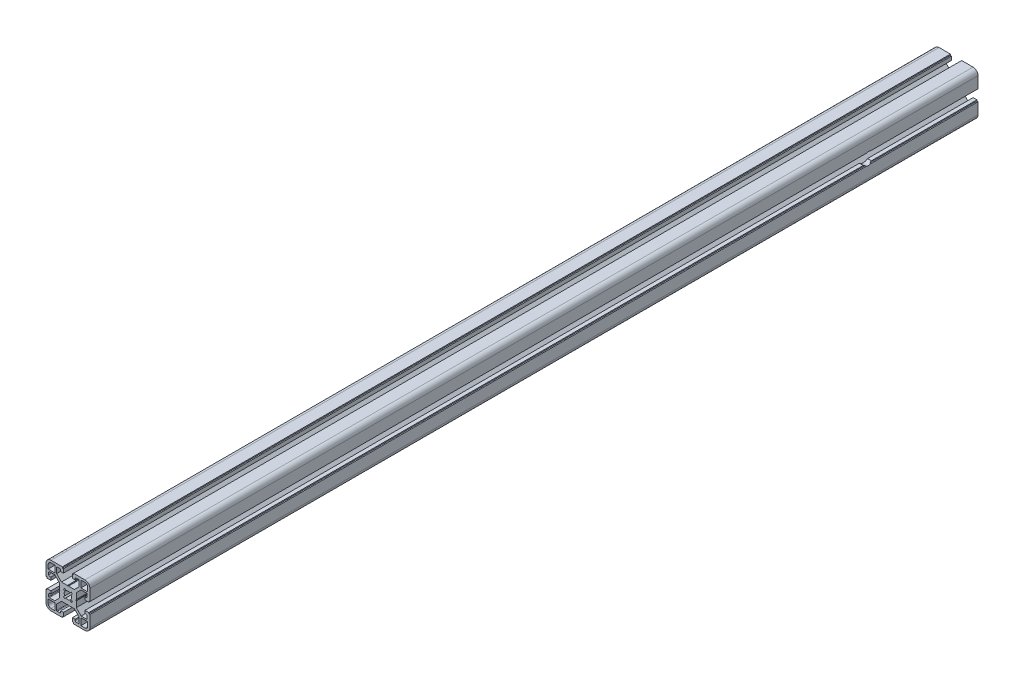
SolidWorks part; units mm, degrees
material "6061 GB/T6892-2006"
ref_plane "前视" through (0, 0, 0) normal (0, 0, 1) x (1, 0, 0)
ref_plane "上视" through (0, 0, 0) normal (0, 1, 0) x (1, 0, 0)
ref_plane "右视" through (0, 0, 0) normal (1, 0, 0) x (0, 0, -1)
sketch "草图1" plane through (0, 0, 0) normal (0, 0, 1) x (1, 0, 0)
  line L0 (-18.9995, -4.1003) -> (-18.9995, -5.1003)
  line L1 (-18.9995, -5.1003) -> (-19.9995, -5.1003)
  line L2 (-19.9995, -5.1003) -> (-19.9995, -15.5003)
  line L3 (-15.4995, -20.0003) -> (-5.0995, -20.0003)
  line L4 (-5.0995, -20.0003) -> (-5.0995, -19.0003)
  line L5 (-5.0995, -19.0003) -> (-4.0995, -19.0003)
  line L6 (-4.0995, -19.0003) -> (-4.0995, -15.5003)
  line L7 (-4.0995, -15.5003) -> (-6.5995, -15.5003)
  line L8 (-6.5995, -15.5003) -> (-6.5995, -16.5003)
  line L9 (-7.5995, -17.5003) -> (-9.7995, -17.5003)
  line L10 (-10.2995, -17.0003) -> (-10.2995, -11.9973)
  line L11 (-10.2995, -11.9973) -> (-5.9025, -7.6003)
  line L12 (-5.9025, -7.6003) -> (-0.5195, -7.6003)
  line L13 (-0.5195, -7.6003) -> (0.0005, -7.3003)
  line L14 (0.0005, -7.3003) -> (0.5195, -7.6003)
  line L15 (0.5195, -7.6003) -> (5.9035, -7.6003)
  line L16 (5.9035, -7.6003) -> (10.3005, -11.9973)
  line L17 (10.3005, -11.9973) -> (10.3005, -17.0003)
  line L18 (9.8005, -17.5003) -> (7.6005, -17.5003)
  line L19 (6.6005, -16.5003) -> (6.6005, -15.5003)
  line L20 (6.6005, -15.5003) -> (4.1005, -15.5003)
  line L21 (4.1005, -15.5003) -> (4.1005, -19.0003)
  line L22 (4.1005, -19.0003) -> (5.1005, -19.0003)
  line L23 (5.1005, -19.0003) -> (5.1005, -20.0003)
  line L24 (5.1005, -20.0003) -> (15.5005, -20.0003)
  line L25 (20.0005, -15.5003) -> (20.0005, -5.1003)
  line L26 (20.0005, -5.1003) -> (19.0005, -5.1003)
  line L27 (19.0005, -5.1003) -> (19.0005, -4.1003)
  line L28 (19.0005, -4.1003) -> (15.5005, -4.1003)
  line L29 (15.5005, -4.1003) -> (15.5005, -6.6003)
  line L30 (15.5005, -6.6003) -> (16.5005, -6.6003)
  line L31 (17.5005, -7.6003) -> (17.5005, -9.8003)
  line L32 (17.0005, -10.3003) -> (11.9975, -10.3003)
  line L33 (11.9975, -10.3003) -> (7.6005, -5.9033)
  line L34 (7.6005, -5.9033) -> (7.6005, -0.5203)
  line L35 (7.6005, -0.5203) -> (7.3005, -0.0003)
  line L36 (7.3005, -0.0003) -> (7.6005, 0.5197)
  line L37 (7.6005, 0.5197) -> (7.6005, 5.9027)
  line L38 (7.6005, 5.9027) -> (11.9975, 10.2997)
  line L39 (11.9975, 10.2997) -> (17.0005, 10.2997)
  line L40 (17.5005, 9.7997) -> (17.5005, 7.5997)
  line L41 (16.5005, 6.5997) -> (15.5005, 6.5997)
  line L42 (15.5005, 6.5997) -> (15.5005, 4.0997)
  line L43 (15.5005, 4.0997) -> (19.0005, 4.0997)
  line L44 (19.0005, 4.0997) -> (19.0005, 5.0997)
  line L45 (19.0005, 5.0997) -> (20.0005, 5.0997)
  line L46 (20.0005, 5.0997) -> (20.0005, 15.4997)
  line L47 (15.5005, 19.9997) -> (5.1005, 19.9997)
  line L48 (5.1005, 19.9997) -> (5.1005, 18.9997)
  line L49 (5.1005, 18.9997) -> (4.1005, 18.9997)
  line L50 (4.1005, 18.9997) -> (4.1005, 15.4997)
  line L51 (4.1005, 15.4997) -> (6.6005, 15.4997)
  line L52 (7.6005, 17.4997) -> (9.8005, 17.4997)
  line L53 (10.3005, 16.9997) -> (10.3005, 11.9967)
  line L54 (10.3005, 11.9967) -> (5.9035, 7.5997)
  line L55 (5.9035, 7.5997) -> (0.5195, 7.5997)
  line L56 (0.5195, 7.5997) -> (0.0005, 7.2997)
  line L57 (0.0005, 7.2997) -> (-0.5195, 7.5997)
  line L58 (-0.5195, 7.5997) -> (-5.9025, 7.5997)
  line L59 (-5.9025, 7.5997) -> (-10.2995, 11.9967)
  line L60 (-10.2995, 11.9967) -> (-10.2995, 16.9997)
  line L61 (-9.7995, 17.4997) -> (-7.5995, 17.4997)
  line L62 (-6.5995, 16.4997) -> (-6.5995, 15.4997)
  line L63 (-6.5995, 15.4997) -> (-4.0995, 15.4997)
  line L64 (-4.0995, 15.4997) -> (-4.0995, 18.9997)
  line L65 (-4.0995, 18.9997) -> (-5.0995, 18.9997)
  line L66 (-5.0995, 18.9997) -> (-5.0995, 19.9997)
  line L67 (-5.0995, 19.9997) -> (-15.4995, 19.9997)
  line L68 (-19.9995, 15.4997) -> (-19.9995, 5.0997)
  line L69 (-19.9995, 5.0997) -> (-18.9995, 5.0997)
  line L70 (-18.9995, 5.0997) -> (-18.9995, 4.0997)
  line L71 (-18.9995, 4.0997) -> (-15.4995, 4.0997)
  line L72 (-15.4995, 4.0997) -> (-15.4995, 6.5997)
  line L73 (-15.4995, 6.5997) -> (-16.4995, 6.5997)
  line L74 (-17.4995, 7.5997) -> (-17.4995, 9.7997)
  line L75 (-16.9995, 10.2997) -> (-11.9965, 10.2997)
  line L76 (-11.9965, 10.2997) -> (-7.5995, 5.9027)
  line L77 (-7.5995, 5.9027) -> (-7.5995, 0.5197)
  line L78 (-7.5995, 0.5197) -> (-7.2995, -0.0003)
  line L79 (-7.2995, -0.0003) -> (-7.5995, -0.5203)
  line L80 (-7.5995, -0.5203) -> (-7.5995, -5.9033)
  line L81 (-7.5995, -5.9033) -> (-11.9965, -10.3003)
  line L82 (-11.9965, -10.3003) -> (-16.9995, -10.3003)
  line L83 (-17.4995, -9.8003) -> (-17.4995, -7.6003)
  line L84 (-16.4995, -6.6003) -> (-15.4995, -6.6003)
  line L85 (-15.4995, -6.6003) -> (-15.4995, -4.1003)
  line L86 (-15.4995, -4.1003) -> (-18.9995, -4.1003)
  line L87 (15.5005, -18.0003) -> (11.8005, -18.0003)
  line L88 (11.8005, -18.0003) -> (11.8005, -11.8003)
  line L89 (11.8005, -11.8003) -> (18.0005, -11.8003)
  line L90 (18.0005, -11.8003) -> (18.0005, -15.5003)
  line L91 (18.0005, 11.7997) -> (11.8005, 11.7997)
  line L92 (11.8005, 11.7997) -> (11.8005, 17.9997)
  line L93 (11.8005, 17.9997) -> (15.5005, 17.9997)
  line L94 (18.0005, 15.4997) -> (18.0005, 11.7997)
  line L95 (-1.8145, -2.8753) -> (-3.0044, -4.0665)
  line L96 (-3.0044, -4.0665) -> (-4.0656, -3.0052)
  line L97 (-4.0656, -3.0052) -> (-2.8745, -1.8153)
  line L98 (-2.8745, 1.8147) -> (-4.0644, 3.0058)
  line L99 (-4.0644, 3.0058) -> (-3.0044, 4.0658)
  line L100 (-3.0044, 4.0658) -> (-1.8145, 2.8747)
  line L101 (1.8145, 2.8747) -> (3.0055, 4.0657)
  line L102 (3.0055, 4.0657) -> (4.0666, 3.0045)
  line L103 (4.0666, 3.0045) -> (2.8755, 1.8147)
  line L104 (2.8755, -1.8153) -> (4.0666, -3.0052)
  line L105 (4.0666, -3.0052) -> (3.0055, -4.0663)
  line L106 (3.0055, -4.0663) -> (1.8145, -2.8753)
  line L107 (-17.9995, -15.5003) -> (-17.9995, -11.8003)
  line L108 (-17.9995, -11.8003) -> (-11.7995, -11.8003)
  line L109 (-11.7995, -11.8003) -> (-11.7995, -18.0003)
  line L110 (-11.7995, -18.0003) -> (-15.4995, -18.0003)
  line L111 (-11.7995, 17.9997) -> (-11.7995, 11.7997)
  line L112 (-11.7995, 11.7997) -> (-17.9995, 11.7997)
  line L113 (-17.9995, 11.7997) -> (-17.9995, 15.4997)
  line L114 (-15.4995, 17.9997) -> (-11.7995, 17.9997)
  arc A0 (-19.9995, -15.5003) -> (-15.4995, -20.0003) centre (-15.4995, -15.5003) ccw
  arc A1 (-6.5995, -16.5003) -> (-7.5995, -17.5003) centre (-7.5995, -16.5003) cw
  arc A2 (-9.7995, -17.5003) -> (-10.2995, -17.0003) centre (-9.7995, -17.0003) cw
  arc A3 (10.3005, -17.0003) -> (9.8005, -17.5003) centre (9.8005, -17.0003) cw
  arc A4 (7.6005, -17.5003) -> (6.6005, -16.5003) centre (7.6005, -16.5003) cw
  arc A5 (15.5005, -20.0003) -> (20.0005, -15.5003) centre (15.5005, -15.5003) ccw
  arc A6 (16.5005, -6.6003) -> (17.5005, -7.6003) centre (16.5005, -7.6003) cw
  arc A7 (17.5005, -9.8003) -> (17.0005, -10.3003) centre (17.0005, -9.8003) cw
  arc A8 (17.0005, 10.2997) -> (17.5005, 9.7997) centre (17.0005, 9.7997) cw
  arc A9 (17.5005, 7.5997) -> (16.5005, 6.5997) centre (16.5005, 7.5997) cw
  arc A10 (20.0005, 15.4997) -> (15.5005, 19.9997) centre (15.5005, 15.4997) ccw
  arc A11 (6.6005, 15.4997) -> (6.6005, 16.4997) centre (7.1003, 15.9997) cw
  arc A12 (6.6005, 16.4997) -> (7.6005, 17.4997) centre (7.6005, 16.4997) cw
  arc A13 (9.8005, 17.4997) -> (10.3005, 16.9997) centre (9.8005, 16.9997) cw
  arc A14 (-10.2995, 16.9997) -> (-9.7995, 17.4997) centre (-9.7995, 16.9997) cw
  arc A15 (-7.5995, 17.4997) -> (-6.5995, 16.4997) centre (-7.5995, 16.4997) cw
  arc A16 (-15.4995, 19.9997) -> (-19.9995, 15.4997) centre (-15.4995, 15.4997) ccw
  arc A17 (-16.4995, 6.5997) -> (-17.4995, 7.5997) centre (-16.4995, 7.5997) cw
  arc A18 (-17.4995, 9.7997) -> (-16.9995, 10.2997) centre (-16.9995, 9.7997) cw
  arc A19 (-16.9995, -10.3003) -> (-17.4995, -9.8003) centre (-16.9995, -9.8003) cw
  arc A20 (-17.4995, -7.6003) -> (-16.4995, -6.6003) centre (-16.4995, -7.6003) cw
  arc A21 (18.0005, -15.5003) -> (15.5005, -18.0003) centre (15.5005, -15.5003) cw
  arc A22 (15.5005, 17.9997) -> (18.0005, 15.4997) centre (15.5005, 15.4997) cw
  arc A23 (-2.8745, -1.8153) -> (-2.8745, 1.8147) centre (0.0005, -0.0003) cw
  arc A24 (-1.8145, 2.8747) -> (1.8145, 2.8747) centre (0, -0.0007) cw
  arc A25 (2.8755, 1.8147) -> (2.8755, -1.8153) centre (0.0005, -0.0003) cw
  arc A26 (1.8145, -2.8753) -> (-1.8145, -2.8753) centre (0, 0) cw
  arc A27 (-15.4995, -18.0003) -> (-17.9995, -15.5003) centre (-15.4995, -15.5003) cw
  arc A28 (-17.9995, 15.4997) -> (-15.4995, 17.9997) centre (-15.4995, 15.4997) cw
extrude "凸台-拉伸1" add sketch "草图1" against normal blind 810
hole_wizard "打孔尺寸(%根据)内六角圆柱头螺钉的类型2" positions "草图2" profile "草图3" counterbore size "M6" standard "GB"
sketch "草图2" plane through (20.0005, 0, 0) normal (1, 0, 0) x (0, 0, -1)
  line L0 (810, -0.0003) -> (0, -0.0003) construction
  point P0 (710, -0.0003)
  dimension "D1" = 100
sketch "草图3" plane through (20.0005, -0.0003, -710) normal (0, 1, 0) x (0, 0, -1)
  line L0 (0, 0) -> (0, 21.9828)
  line L1 (0, 21.9828) -> (3.3, 20)
  line L2 (3.3, 20) -> (3.3, 6.8)
  line L3 (3.3, 6.8) -> (5.5, 6.8)
  line L4 (5.5, 6.8) -> (5.5, 0)
  line L5 (5.5, 0) -> (0, 0)
  line L10 (0, 21.9828) -> (-3.3, 20) construction
  line L11 (0, -6.35) -> (0, 107.95) construction
  dimension "孔直径" = 6.6
  dimension "孔深度" = 20
  dimension "柱形沉头孔直径" = 11
  dimension "柱形沉头孔深度" = 6.8
  dimension "导头角度" = 118
hole_wizard "打孔尺寸(%根据)内六角圆柱头螺钉的类型2" positions "草图4" profile "草图5" counterbore size "M6" standard "GB"
sketch "草图4" plane through (-19.9995, 0, 0) normal (-1, 0, 0) x (0, 0, 1)
  line L0 (-810, -0.0003) -> (0, -0.0003) construction
  point P0 (-710, -0.0003)
  dimension "D1" = 100
sketch "草图5" plane through (-19.9995, -0.0003, -710) normal (0, 1, 0) x (0, 0, 1)
  line L0 (0, 0) -> (0, 21.9828)
  line L1 (0, 21.9828) -> (3.3, 20)
  line L2 (3.3, 20) -> (3.3, 6.8)
  line L3 (3.3, 6.8) -> (5.5, 6.8)
  line L4 (5.5, 6.8) -> (5.5, 0)
  line L5 (5.5, 0) -> (0, 0)
  line L10 (0, 21.9828) -> (-3.3, 20) construction
  line L11 (0, -6.35) -> (0, 107.95) construction
  dimension "孔直径" = 6.6
  dimension "孔深度" = 20
  dimension "柱形沉头孔直径" = 11
  dimension "柱形沉头孔深度" = 6.8
  dimension "导头角度" = 118
